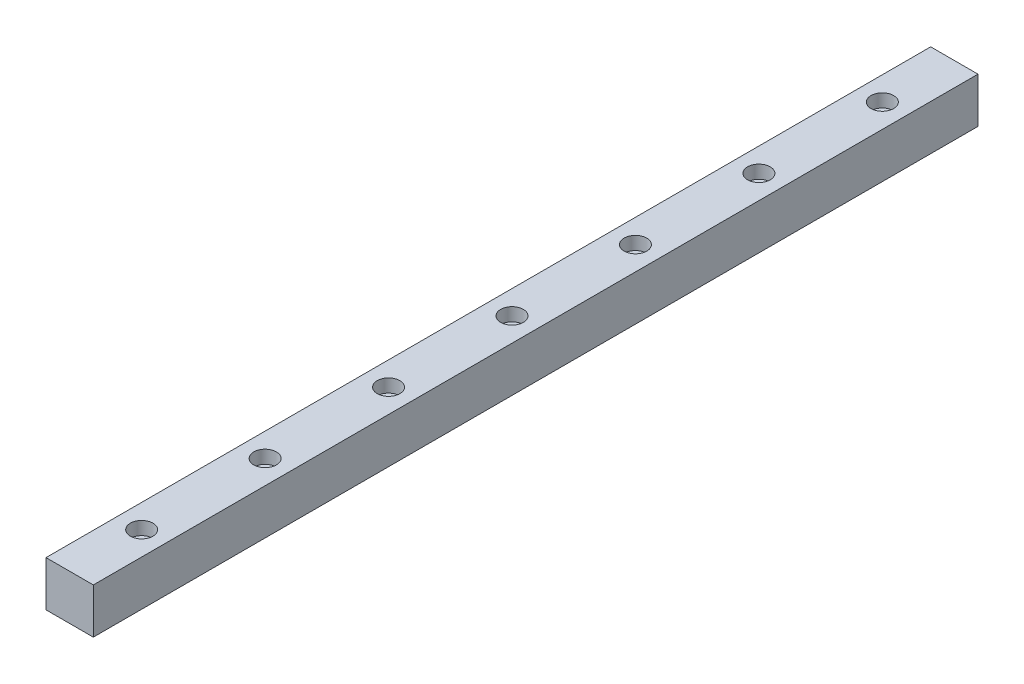
SolidWorks part; units mm, degrees
ref_plane "前视基准面" through (0, 0, 0) normal (0, 0, 1) x (1, 0, 0)
ref_plane "上视基准面" through (0, 0, 0) normal (0, 1, 0) x (1, 0, 0)
ref_plane "右视基准面" through (0, 0, 0) normal (1, 0, 0) x (0, 0, -1)
sketch "草图1" plane through (0, 0, 0) normal (0, 0, 1) x (1, 0, 0)
  line L1 (0, 0) -> (23, 0)
  line L2 (0, 0) -> (0, 22)
  line L3 (0, 22) -> (23, 22)
  line L4 (23, 0) -> (23, 22)
  dimension "D1" = 23
  dimension "D2" = 22
extrude "凸台-拉伸1" add sketch "草图1" along normal blind 430
hole_wizard "M6 六角凹头螺钉的柱形沉头孔1" positions "草图3" profile "草图2" counterbore size "M6" standard "ISO" end condition through all
sketch "草图3" plane through (0, 22, 0) normal (0, 1, 0) x (1, 0, 0)
  line L3 (11.5, -430) -> (11.5, -368.7517) construction
  line L4 (23, -430) -> (0, -430) construction
  point P0 (11.5, -395)
  dimension "D1" = 35
sketch "草图2" plane through (11.5, 22, 395) normal (1, 0, 0) x (0, 0, 1)
  line L0 (0, 0) -> (0, 22)
  line L1 (0, 22) -> (3.3, 22)
  line L3 (3.3, 22) -> (3.3, 6.4)
  line L4 (3.3, 6.4) -> (5.5, 6.4)
  line L5 (5.5, 6.4) -> (5.5, 0)
  line L7 (5.5, 0) -> (0, 0)
  line L11 (0, -6.35) -> (0, 107.95) construction
  dimension "通孔孔直径" = 6.6
  dimension "通孔孔深度" = 22
  dimension "柱形沉头孔直径" = 11
  dimension "柱形沉头孔深度" = 6.4
pattern_linear "阵列(线性)1" count 7 spacing 60 along (0, 0, -1) of "M6 六角凹头螺钉的柱形沉头孔1"
